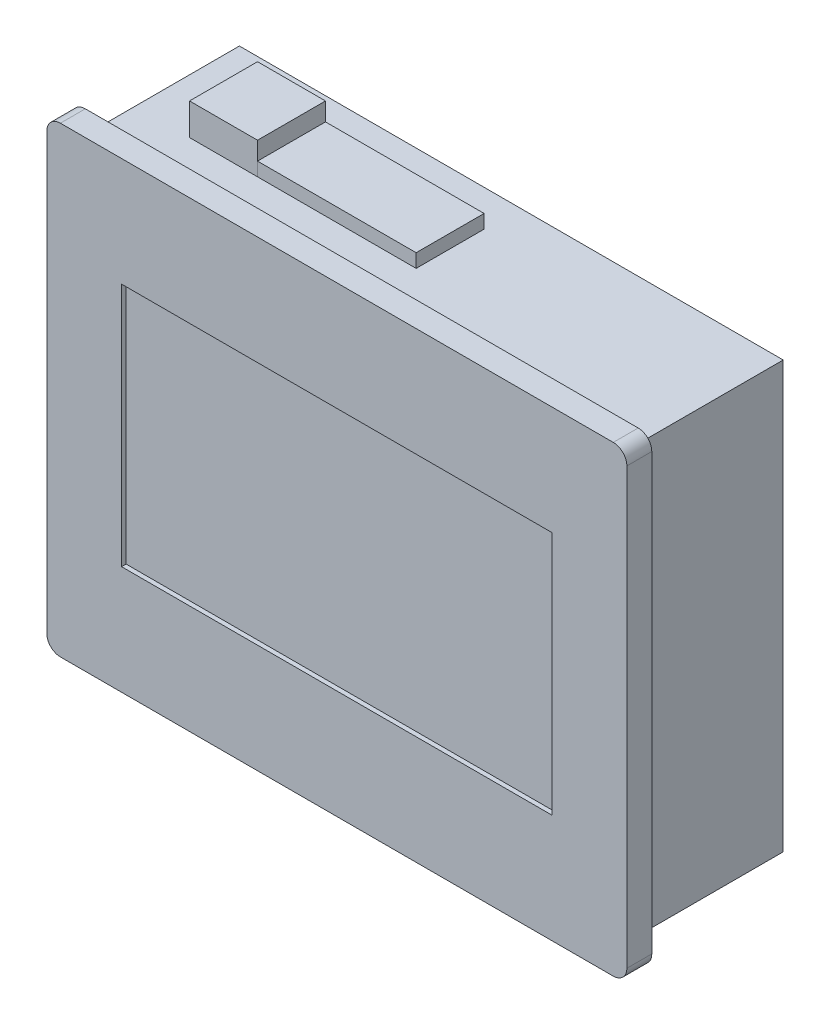
from build123d import *

# Parameters (mm, degrees)
SKETCH1_W           = 128
SKETCH1_H           = 102
BOSS_EXTRUDE1_DEPTH = 5.5
SKETCH2_W           = 95
SKETCH2_H           = 54
CUT_EXTRUDE1_DEPTH  = 1
SKETCH3_W           = 120
SKETCH3_H           = 94
BOSS_EXTRUDE2_DEPTH = 33
FILLET1_R           = 3
SKETCH4_W           = 15
SKETCH4_H           = 15
BOSS_EXTRUDE3_DEPTH = 7
SKETCH5_W           = 35
SKETCH5_H           = 15
BOSS_EXTRUDE4_DEPTH = 3


with BuildPart() as part:
    # Sketch1 → Boss-Extrude1 (new body)
    with BuildSketch(Plane.XY):
        Rectangle(SKETCH1_W, SKETCH1_H)
    extrude(amount=BOSS_EXTRUDE1_DEPTH)

    # Sketch2 → Cut-Extrude1 (cut)
    with BuildSketch(Plane.XY.offset(5.5)):
        Rectangle(SKETCH2_W, SKETCH2_H)
    extrude(amount=-CUT_EXTRUDE1_DEPTH, mode=Mode.SUBTRACT)

    # Sketch3 → Boss-Extrude2 (add)
    with BuildSketch(Plane(origin=(0, 0, 0), x_dir=(-1, 0, 0), z_dir=(0, 0, -1))):
        Rectangle(SKETCH3_W, SKETCH3_H)
    extrude(amount=BOSS_EXTRUDE2_DEPTH)

    # Fillet1
    fillet1_edges = [part.edges().sort_by_distance(p)[0] for p in [
        (-64, 51, 2.75),
        (64, 51, 2.75),
        (64, -51, 2.75),
        (-64, -51, 2.75),
    ]]
    fillet(fillet1_edges, radius=FILLET1_R)

    # Sketch4 → Boss-Extrude3 (add)
    with BuildSketch(Plane(origin=(0, 47, 0), x_dir=(1, 0, 0), z_dir=(0, 1, 0))):
        with Locations((-40.5, 17.5)):
            Rectangle(SKETCH4_W, SKETCH4_H)
    extrude(amount=BOSS_EXTRUDE3_DEPTH)


with BuildPart() as body_2:
    # Sketch5 → Boss-Extrude4 (new body)
    with BuildSketch(Plane(origin=(0, 47, 0), x_dir=(1, 0, 0), z_dir=(0, 1, 0))):
        with Locations((-15.5, 17.5)):
            Rectangle(SKETCH5_W, SKETCH5_H)
    extrude(amount=BOSS_EXTRUDE4_DEPTH)


solid = Compound([part.part, body_2.part])
